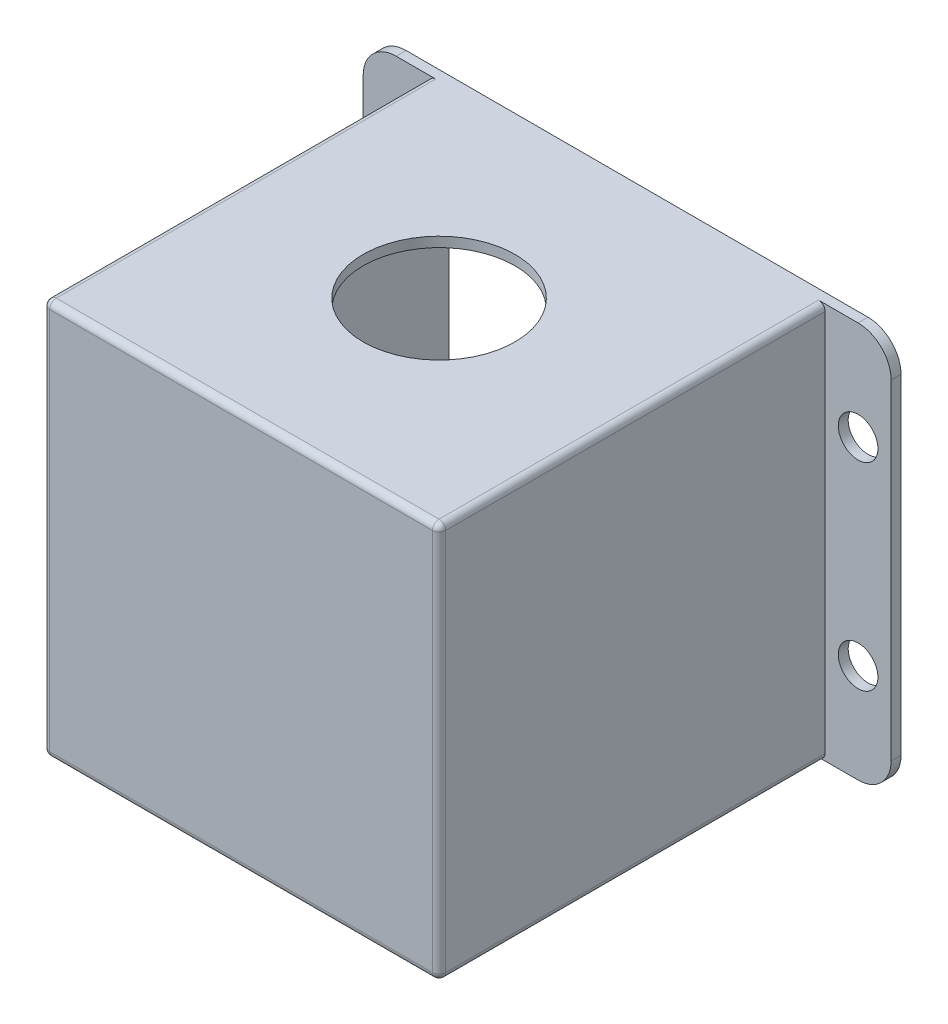
from build123d import *

# Parameters (mm, degrees)
SKETCH_1_W          = 60
SKETCH_1_H          = 60
EXTRUDE_1_DEPTH     = 30
SHELL_1_T           = -1.5
SKETCH_5_W          = 1.5
SKETCH_5_H          = 60
EXTRUDE_3_DEPTH     = 10
SKETCH_6_W          = 1.5
SKETCH_6_H          = 60
EXTRUDE_4_DEPTH     = 10
CUT_EXTRUDE_3_REACH = 80.102
SKETCH_7_W          = 20
SKETCH_7_H          = 15
FILLET_1_R          = 5
FILLET_2_R          = 5
CUT_EXTRUDE_4_REACH = 80.102
SKETCH_8_R          = 11.5
FILLET_3_R          = 1
SKETCH_9_R          = 3
CUT_EXTRUDE_5_DEPTH = 77.956156349


with BuildPart() as part:
    # 草图1 → 凸台-拉伸1 (new, symmetric)
    with BuildSketch(Plane.XY):
        Rectangle(SKETCH_1_W, SKETCH_1_H)
    extrude(amount=EXTRUDE_1_DEPTH, both=True)

    # 抽壳1
    shell_1_openings = [part.faces().sort_by_distance(p)[0] for p in [
        (0, 0, -30),
    ]]
    offset(amount=SHELL_1_T, openings=shell_1_openings, kind=Kind.INTERSECTION)

    # 草图5 → 凸台-拉伸3 (add)
    with BuildSketch(Plane(origin=(30, 0, 0), x_dir=(0, 0, -1), z_dir=(1, 0, 0))):
        with Locations((29.25, 0)):
            Rectangle(SKETCH_5_W, SKETCH_5_H)
    extrude(amount=EXTRUDE_3_DEPTH)

    # 草图6 → 凸台-拉伸4 (add)
    with BuildSketch(Plane.ZY.offset(30)):
        with Locations((-29.25, 0)):
            Rectangle(SKETCH_6_W, SKETCH_6_H)
    extrude(amount=EXTRUDE_4_DEPTH)

    # 草图7 → 切除-拉伸3 (cut, up to next)
    with BuildSketch(Plane.XZ.offset(30), mode=Mode.PRIVATE) as cut_extrude_3_sk1:
        with Locations((0, -22.5)):
            Rectangle(SKETCH_7_W, SKETCH_7_H)
    cut_extrude_3_tool1 = extrude(cut_extrude_3_sk1.sketch, amount=-CUT_EXTRUDE_3_REACH, mode=Mode.PRIVATE) & part.part
    add(cut_extrude_3_tool1.solids().sort_by_distance((0, -30, -22.5))[0], mode=Mode.SUBTRACT)

    # 圆角1
    fillet_1_edges = [part.edges().sort_by_distance(p)[0] for p in [
        (10, -29.25, -15),
        (-10, -29.25, -15),
    ]]
    fillet(fillet_1_edges, radius=FILLET_1_R)

    # 圆角2
    fillet_2_edges = [part.edges().sort_by_distance(p)[0] for p in [
        (40, 30, -29.25),
        (40, -30, -29.25),
        (-40, -30, -29.25),
        (-40, 30, -29.25),
    ]]
    fillet(fillet_2_edges, radius=FILLET_2_R)

    # 草图8 → 切除-拉伸4 (cut, up to next)
    with BuildSketch(Plane(origin=(0, 30, 0), x_dir=(1, 0, 0), z_dir=(0, 1, 0)), mode=Mode.PRIVATE) as cut_extrude_4_sk1:
        with Locations(Location((0, 0, 0), (0, 0, 270))):
            Circle(SKETCH_8_R)
    cut_extrude_4_tool1 = extrude(cut_extrude_4_sk1.sketch, amount=-CUT_EXTRUDE_4_REACH, mode=Mode.PRIVATE) & part.part
    add(cut_extrude_4_tool1.solids().sort_by_distance((0, 30, 0))[0], mode=Mode.SUBTRACT)

    # 圆角3
    fillet_3_edges = [part.edges().sort_by_distance(p)[0] for p in [
        (-30, 0, 30),
        (0, -30, 30),
        (30, 0, 30),
        (0, 30, 30),
        (30, -30, 0.75),
        (-30, -30, 0.75),
        (-30, 30, 0.75),
        (30, 30, 0.75),
    ]]
    fillet(fillet_3_edges, radius=FILLET_3_R)

    # 草图9 → 切除-拉伸5 (cut, through all)
    with BuildSketch(Plane.XY.offset(-28.5)):
        with Locations((35, -15)):
            Circle(SKETCH_9_R)
        with Locations((35, 15)):
            Circle(SKETCH_9_R)
    cut_extrude_5 = extrude(amount=-CUT_EXTRUDE_5_DEPTH, mode=Mode.SUBTRACT)

    # 镜向1: 切除-拉伸5 across plane
    add(cut_extrude_5.mirror(Plane(origin=(0, 0, 0), x_dir=(0, 0, 1), z_dir=(1, 0, 0))), mode=Mode.SUBTRACT)


solid = part.part
